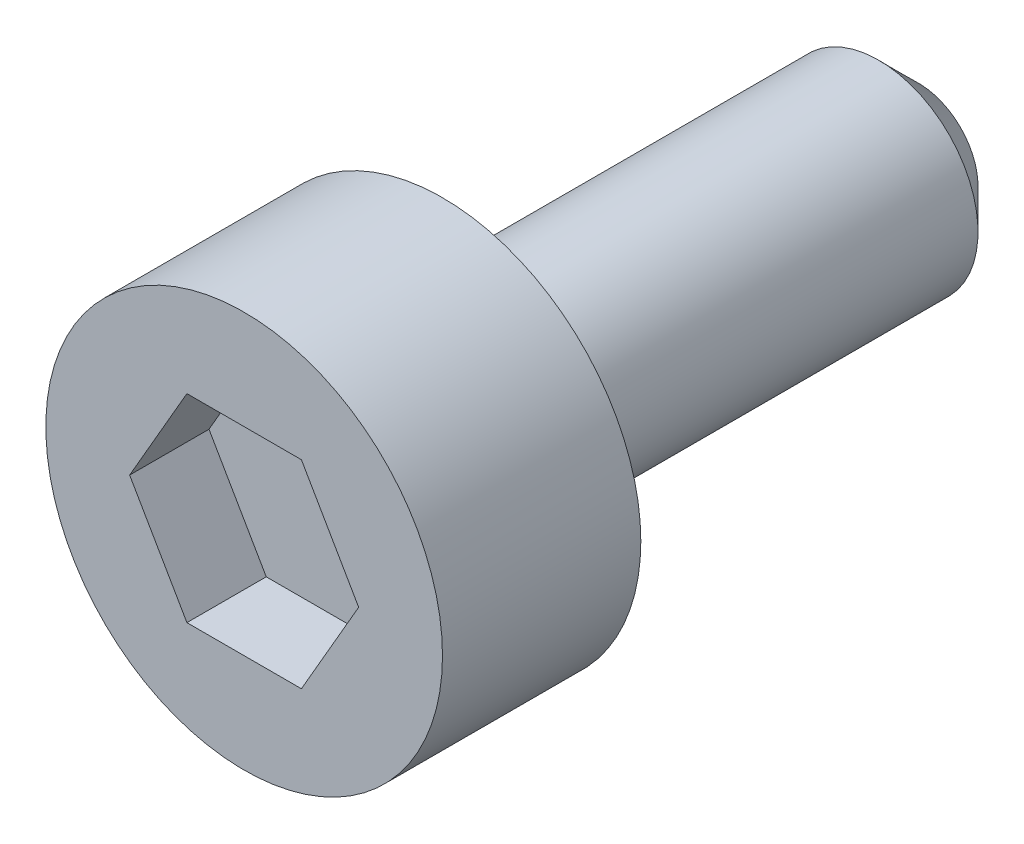
SolidWorks part; units mm, degrees
ref_plane "Front Plane" through (0, 0, 0) normal (0, 0, 1) x (1, 0, 0)
ref_plane "Top Plane" through (0, 0, 0) normal (0, 1, 0) x (1, 0, 0)
ref_plane "Right Plane" through (0, 0, 0) normal (1, 0, 0) x (0, 0, -1)
other "Configuration Table"
sketch "Sketch1" plane through (0, 0, 0) normal (0, 0, 1) x (1, 0, 0)
  circle A0 centre (0, 0) radius 5
  dimension "D1" = 10
extrude "Boss-Extrude1" add sketch "Sketch1" along normal blind 5
sketch "Sketch2" plane through (0, 0, 5) normal (0, 0, 1) x (1, 0, 0)
  line L1 (2.8868, 0) -> (1.4434, 2.5)
  line L2 (1.4434, 2.5) -> (-1.4434, 2.5)
  line L3 (-1.4434, 2.5) -> (-2.8868, 0)
  line L4 (-2.8868, 0) -> (-1.4434, -2.5)
  line L5 (-1.4434, -2.5) -> (1.4434, -2.5)
  line L6 (1.4434, -2.5) -> (2.8868, 0)
  circle A0 centre (0, 0) radius 2.5 construction
  dimension "D1" = 5
extrude "Cut-Extrude1" cut sketch "Sketch2" against normal blind 2
sketch "Sketch3" plane through (0, 0, 0) normal (0, 0, -1) x (-1, 0, 0)
  circle A0 centre (0, 0) radius 2.5
  dimension "D1" = 5
extrude "Boss-Extrude2" add sketch "Sketch3" along normal blind 12
chamfer "Chamfer1" distance 1 angle 45 1 edges at (-2.5, 0, -12)
